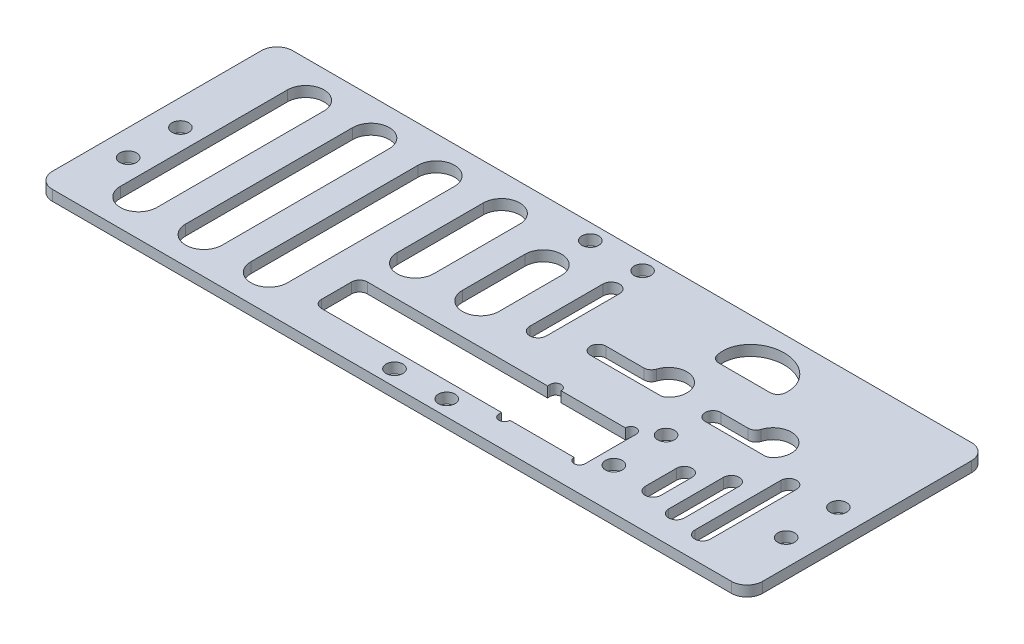
SolidWorks part; units mm, degrees
material "Thornel Mat VMA"
ref_plane "前视基准面" through (0, 0, 0) normal (0, 0, 1) x (1, 0, 0)
ref_plane "上视基准面" through (0, 0, 0) normal (0, 1, 0) x (1, 0, 0)
ref_plane "右视基准面" through (0, 0, 0) normal (1, 0, 0) x (0, 0, -1)
sketch "草图1" plane through (0, 0, 0) normal (0, 1, 0) x (1, 0, 0)
  line L0 (0, 23) -> (0, -23) construction
  line L1 (68, -23) -> (-68, -23)
  line L2 (68, -23) -> (68, 23)
  line L3 (68, 23) -> (-68, 23)
  line L4 (-68, -23) -> (-68, 23)
  line L5 (68, -23) -> (-68, 23) construction
  line L6 (68, 23) -> (-68, -23) construction
  line L7 (-63, -0.5) -> (-63, -10.5) construction
  line L8 (-2.5, -20) -> (7.5, -20) construction
  line L9 (34.5, -5) -> (34.5, -15) construction
  line L10 (63, -0.5) -> (63, -10.5) construction
  line L11 (-68, 0) -> (68, 0) construction
  line L12 (5, 20) -> (-5, 20) construction
  circle A0 centre (-63, -0.5) radius 1.6
  circle A1 centre (-63, -10.5) radius 1.6
  circle A2 centre (-2.5, -20) radius 1.6
  circle A3 centre (7.5, -20) radius 1.6
  circle A6 centre (63, -10.5) radius 1.6
  circle A7 centre (63, -0.5) radius 1.6
  circle A8 centre (5, 20) radius 1.6
  circle A9 centre (-5, 20) radius 1.6
  circle A12 centre (34.5, -5) radius 1.6
  circle A13 centre (34.5, -15) radius 1.6
  point P0 (0, 0)
  dimension "D2" = 12.5
  dimension "D4" = 3.2
  dimension "D11" = 33.5
  dimension "D1" = 136
  dimension "D3" = 10
  dimension "D5" = 5
  dimension "D6" = 3
  dimension "D7" = 46
  dimension "D8" = 3
  dimension "D10" = 65.5
  dimension "D12" = 8
extrude "凸台-拉伸1" add sketch "草图1" along normal blind 2
sketch "草图2" plane through (0, 2, 0) normal (0, 1, 0) x (1, 0, 0)
  line L0 (-68, -23) -> (68, -23) construction
  line L1 (-55.5, 16) -> (-55.5, -16) construction
  line L2 (-52, 16) -> (-52, -16)
  line L3 (17.1, -7.7) -> (29.4, -7.7)
  line L4 (-59, 16) -> (-59, -16)
  line L5 (-68, 0) -> (68, 0) construction
  line L6 (-21, -8.2) -> (-21, -17)
  line L9 (17.1, -17.5) -> (29.4, -17.5)
  line L12 (31.5, -7.7) -> (31.5, -17.5)
  line L15 (-21, -17) -> (15, -17)
  line L18 (15, -17) -> (15, -17.5)
  line L21 (15, -7.7) -> (15, -8.2)
  line L24 (15, -8.2) -> (-21, -8.2)
  line L25 (-68, 23) -> (-68, -23) construction
  line L26 (68, -23) -> (68, 23) construction
  line L27 (-43, 16) -> (-43, -16) construction
  line L28 (-39.5, 16) -> (-39.5, -16)
  line L29 (-46.5, 16) -> (-46.5, -16)
  line L30 (-30.5, 16) -> (-30.5, -16) construction
  line L31 (-27, 16) -> (-27, -16)
  line L32 (-34, 16) -> (-34, -16)
  line L36 (-5.5, 11.5) -> (-5.5, -0.5) construction
  line L37 (-2, 11.5) -> (-2, -0.5)
  line L38 (-9, 11.5) -> (-9, -0.5)
  line L39 (0, 23) -> (0, -23) construction
  line L40 (68, 23) -> (-68, 23) construction
  line L41 (42.5, 4) -> (36, 4)
  line L50 (36, 1) -> (47.8028, 1)
  line L53 (42.5, -15.5) -> (42.5, -9.5) construction
  line L54 (41, -15.5) -> (41, -9.5)
  line L55 (44, -15.5) -> (44, -9.5)
  line L56 (48.5, -17) -> (48.5, -6.5) construction
  line L57 (47, -17) -> (47, -6.5)
  line L58 (50, -17) -> (50, -6.5)
  line L59 (54.5, -18) -> (54.5, -1.5) construction
  line L60 (53, -18) -> (53, -1.5)
  line L61 (56, -18) -> (56, -1.5)
  line L73 (22.5, 4) -> (14, 4)
  line L82 (27.8028, 1) -> (14, 1)
  line L100 (38.5554, 12) -> (26.5554, 12)
  line L107 (31.4548, 8.5039) -> (33.4517, 19.8292) construction
  line L108 (5, 0) -> (5, 14) construction
  line L109 (3.4, 0) -> (3.4, 14)
  line L110 (6.6, 0) -> (6.6, 14)
  line L111 (26.052, 15.2952) -> (38.8545, 13.0378) construction
  line L112 (-18, -0.5) -> (-18, 16) construction
  line L113 (-21.5, -0.5) -> (-21.5, 16)
  line L114 (-14.5, -0.5) -> (-14.5, 16)
  circle A18 centre (34.5, -15) radius 1.6 construction
  arc A19 (31.5, -7.7) -> (29.4, -7.7) centre (30.45, -7.7) ccw
  arc A20 (29.4, -17.5) -> (31.5, -17.5) centre (30.45, -17.5) ccw
  arc A21 (17.1, -7.7) -> (15, -7.7) centre (16.05, -7.7) ccw
  arc A22 (15, -17.5) -> (17.1, -17.5) centre (16.05, -17.5) ccw
  arc A23 (-52, 16) -> (-59, 16) centre (-55.5, 16) ccw
  arc A24 (-59, -16) -> (-52, -16) centre (-55.5, -16) ccw
  arc A25 (-39.5, 16) -> (-46.5, 16) centre (-43, 16) ccw
  arc A26 (-46.5, -16) -> (-39.5, -16) centre (-43, -16) ccw
  arc A27 (-27, 16) -> (-34, 16) centre (-30.5, 16) ccw
  arc A28 (-34, -16) -> (-27, -16) centre (-30.5, -16) ccw
  arc A31 (-2, 11.5) -> (-9, 11.5) centre (-5.5, 11.5) ccw
  arc A32 (-9, -0.5) -> (-2, -0.5) centre (-5.5, -0.5) ccw
  circle A33 centre (-63, -10.5) radius 1.6 construction
  arc A42 (41, -15.5) -> (44, -15.5) centre (42.5, -15.5) ccw
  arc A43 (44, -9.5) -> (41, -9.5) centre (42.5, -9.5) ccw
  arc A44 (47, -17) -> (50, -17) centre (48.5, -17) ccw
  arc A45 (50, -6.5) -> (47, -6.5) centre (48.5, -6.5) ccw
  arc A46 (53, -18) -> (56, -18) centre (54.5, -18) ccw
  arc A47 (56, -1.5) -> (53, -1.5) centre (54.5, -1.5) ccw
  arc A84 (3.4, 0) -> (6.6, 0) centre (5, 0) ccw
  arc A85 (6.6, 14) -> (3.4, 14) centre (5, 14) ccw
  circle A86 centre (5, 20) radius 1.6 construction
  arc A87 (47.8028, 1) -> (42.5, 4) centre (46, 4) ccw
  arc A88 (36, 4) -> (36, 1) centre (36, 2.5) ccw
  arc A90 (14, 4) -> (14, 1) centre (14, 2.5) ccw
  arc A91 (27.8028, 1) -> (22.5, 4) centre (26, 4) ccw
  arc A92 (-21.5, -0.5) -> (-14.5, -0.5) centre (-18, -0.5) ccw
  arc A93 (-14.5, 16) -> (-21.5, 16) centre (-18, 16) ccw
  circle A94 centre (-5, 20) radius 1.6 construction
  ellipse E0 centre (32.4533, 14.1665) end of major axis (38.8545, 13.0378) minor radius 5.75 (38.5554, 12) -> (26.5554, 12) ccw
  point P21 (-55.5, 0)
  point P35 (-43, 0)
  point P42 (-30.5, 0)
  point P50 (-18, 7.75)
  point P56 (-5.5, 5.5)
  point P69 (5, 7)
  point P84 (0, 0)
  point P91 (-18, 16)
  point P94 (-5.5, 0.6102)
  point P95 (42.5, -12.5)
  point P100 (48.5, -11.75)
  point P109 (54.5, -9.75)
  point P118 (-18, -1.5)
  dimension "D1" = 5.5
  dimension "D4" = 1.05
  dimension "D6" = 0.5
  dimension "D9" = 3.5
  dimension "D15" = 4
  dimension "D16" = 1.5
  dimension "D26" = 3
  dimension "D39" = 12.5
  dimension "D40" = 8.5
  dimension "D49" = 6
  dimension "D27" = 3.5
  dimension "D29" = 12
  dimension "D31" = 22
  dimension "D33" = 11
  dimension "D2" = 9.8
  dimension "D5" = 16.5
  dimension "D7" = 0.5
  dimension "D8" = 36
  dimension "D10" = 32
  dimension "D3" = 3
  dimension "D11" = 3
  dimension "D12" = 12.5
  dimension "D13" = 12.5
  dimension "D14" = 12
  dimension "D17" = 3
  dimension "D18" = 3
  dimension "D19" = 1.5
  dimension "D20" = 1
  dimension "D21" = 5
  dimension "D22" = 3
  dimension "D23" = 6
  dimension "D24" = 8
  dimension "D25" = 5
  dimension "D28" = 10
  dimension "D30" = 10
  dimension "D32" = 22
  dimension "D34" = 12
  dimension "D35" = 35.5467
  dimension "D36" = 10
  dimension "D37" = 11.5
  dimension "D38" = 13
extrude "切除-拉伸1" cut sketch "草图2" against normal through all
fillet "R1.5 镂空圆角" radius 1.5 8 edges at (-21, 1, 8.2) (-21, 1, 17) (38.5554, 1, -12) (26.5554, 1, -12) (22.5, 1, -4) (27.8028, 1, -1) (42.5, 1, -4) (47.8028, 1, -1)
fillet "R3 外缘圆角" radius 3 4 edges at (-68, 1, -23) (68, 1, 23) (-68, 1, 23) (68, 1, -23)
